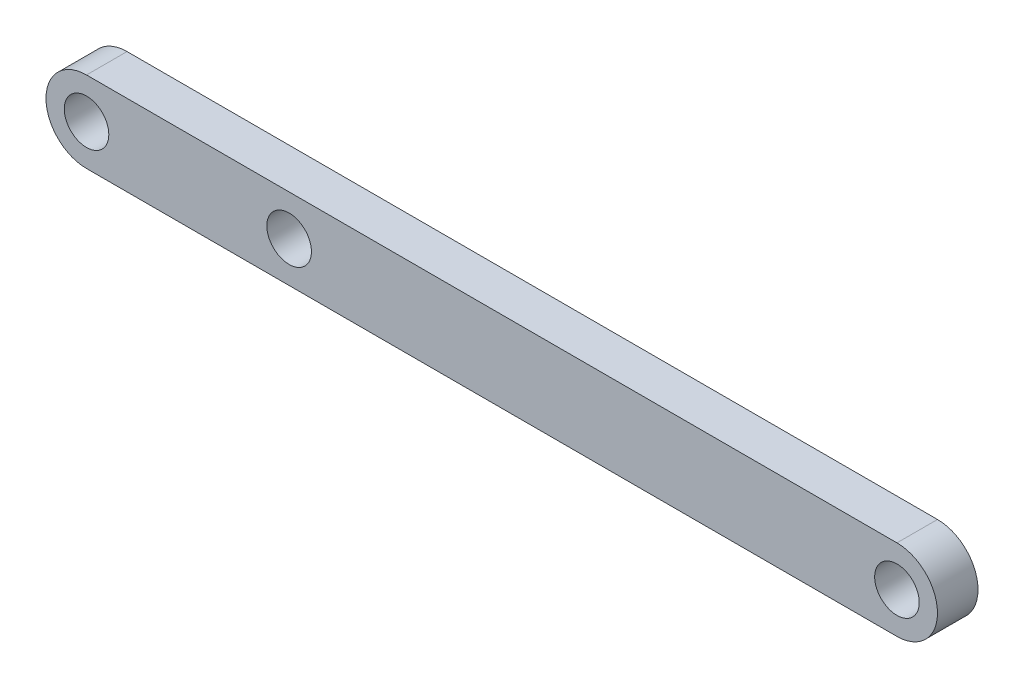
SolidWorks part; units mm, degrees
ref_plane "Alzado" through (0, 0, 0) normal (0, 0, 1) x (1, 0, 0)
ref_plane "Planta" through (0, 0, 0) normal (0, 1, 0) x (1, 0, 0)
ref_plane "Vista lateral" through (0, 0, 0) normal (1, 0, 0) x (0, 0, -1)
sketch "Sketch1" plane through (0, 0, 0) normal (0, 0, 1) x (1, 0, 0)
  line L0 (-10, 0) -> (10, 0) construction
  line L1 (-10, 1) -> (10, 1)
  line L2 (-10, -1) -> (10, -1)
  arc A0 (-10, 1) -> (-10, -1) centre (-10, 0) ccw
  arc A1 (10, -1) -> (10, 1) centre (10, 0) ccw
  circle A2 centre (-10, 0) radius 0.55
  circle A3 centre (10, 0) radius 0.55
  circle A4 centre (-5, 0) radius 0.55
  point P3 (0, 0)
  dimension "D3" = 1.1
  dimension "D4" = 5
  dimension "D1" = 20
  dimension "D2" = 2
extrude "Thigh1 length" add sketch "Sketch1" along normal mid plane 1
sketch "Sketch2" plane through (0, 0, 0.5) normal (0, 0, 1) x (1, 0, 0)
  circle A0 centre (-10, 0) radius 1.8
  circle A1 centre (10, 0) radius 1.8
  circle A2 centre (-5, 0) radius 1.8
  dimension "D1" = 3.6
extrude "Cortar-Extruir1" [suppressed] cut sketch "Sketch2" against normal blind 1
